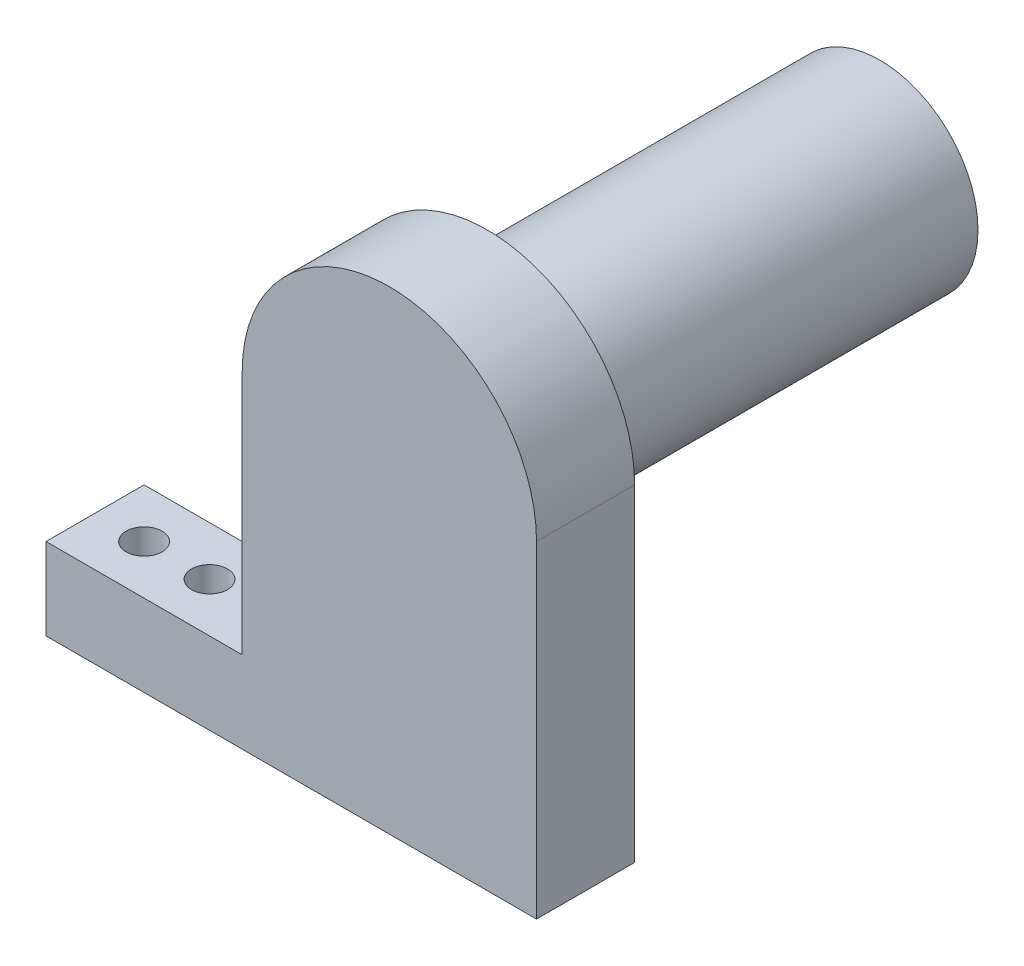
from build123d import *

# Parameters (mm, degrees)
SKETCH2_W           = 150
SKETCH2_H           = 25
BOSS_EXTRUDE1_DEPTH = 15
SKETCH3_R           = 30
BOSS_EXTRUDE2_DEPTH = 30
SKETCH4_R           = 5.5
CUT_EXTRUDE1_DEPTH  = 30
BOSS_EXTRUDE3_START = -30
SKETCH5_R           = 30
BOSS_EXTRUDE3_DEPTH = 150


with BuildPart() as part:
    # Sketch2 → Boss-Extrude1 (new, symmetric)
    with BuildSketch(Plane.XY):
        Rectangle(SKETCH2_W, SKETCH2_H)
    extrude(amount=BOSS_EXTRUDE1_DEPTH, both=True)

    # Sketch3 → Boss-Extrude2 (add)
    with BuildSketch(Plane.XY.offset(15)):
        with BuildLine():
            Line((-15, 87.5), (-15, 0))
            Line((-15, 0), (75, 0))
            Line((75, 0), (75, 87.5))
            ThreePointArc((75, 87.5), (30, 132.5), (-15, 87.5))
        make_face()
        with Locations((30, 87.5)):
            Circle(SKETCH3_R, mode=Mode.SUBTRACT)
    extrude(amount=-BOSS_EXTRUDE2_DEPTH)

    # Sketch4 → Cut-Extrude1 (cut)
    with BuildSketch(Plane(origin=(0, 12.5, 0), x_dir=(1, 0, 0), z_dir=(0, 1, 0))):
        with Locations(Location((-60, 0, 0), (0, 0, 270))):
            Circle(SKETCH4_R)
        with Locations(Location((-40, 0, 0), (0, 0, 270))):
            Circle(SKETCH4_R)
    extrude(amount=-CUT_EXTRUDE1_DEPTH, mode=Mode.SUBTRACT)

    # Sketch5 → Boss-Extrude3 (add)
    with BuildSketch(Plane(origin=(0, 0, -15), x_dir=(-1, 0, 0), z_dir=(0, 0, -1)).offset(BOSS_EXTRUDE3_START)):
        with Locations(Location((-30, 87.5, 0), (0, 0, 180))):
            Circle(SKETCH5_R)
    extrude(amount=BOSS_EXTRUDE3_DEPTH)


solid = part.part
